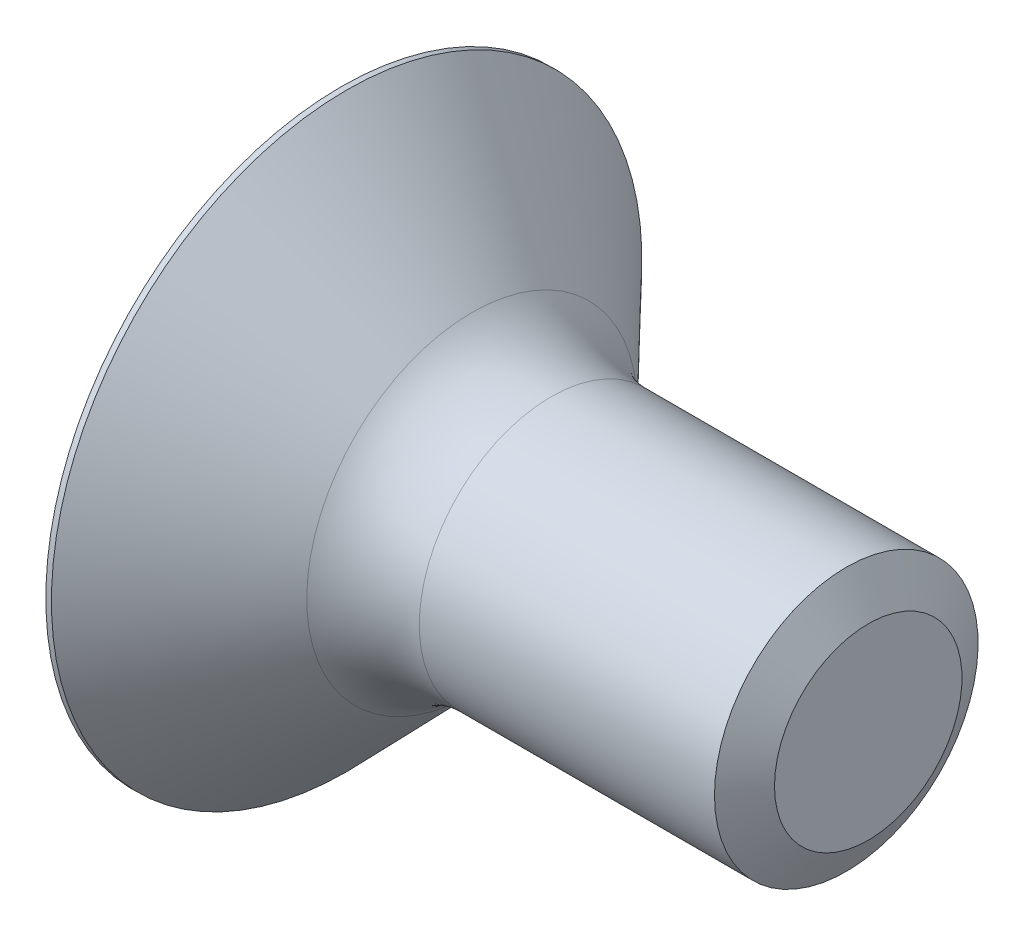
from build123d import *

# Parameters (mm, degrees)
CUT_EXTRUDE1_DEPTH = 3.82


with BuildPart() as part:
    # Sketch1 → Revolve1 (revolve)
    with BuildSketch(Plane.XY):
        with BuildLine():
            Line((0, 3), (-7.218812959, 3))
            ThreePointArc((-7.218812959, 3), (-8.195640781, 3.198737866), (-9.01716246, 3.763354074))
            Line((-9.01716246, 3.763354074), (-11.872362242, 6.72))
            Line((-11.872362242, 6.72), (-12, 6.72))
            Line((-12, 6.72), (-12, 0))
            Line((-12, 0), (0, 0))
            Line((0, 0), (0, 3))
        make_face()
    revolve(axis=Axis((0, 0, 0), (-1, 0, 0)))

    # Sketch2 → Cut-Extrude1 (cut)
    with BuildSketch(Plane.ZY.offset(12)):
        Polygon((0, 2.309401077), (-2, 1.154700538), (-2, -1.154700538), (0, -2.309401077), (2, -1.154700538), (2, 1.154700538), align=None)
    extrude(amount=-CUT_EXTRUDE1_DEPTH, mode=Mode.SUBTRACT)

    # Sketch6 → Revolve2 (revolve)
    with BuildSketch(Plane.XY, mode=Mode.PRIVATE) as revolve2_sk:
        Polygon((-9.8, 2.309401077), (-8.466666667, 0), (-7.6, 0), (-7.6, 2.309401077), align=None)
    revolve(revolve2_sk.sketch.rotate(Axis((-12, 0, 0), (1, 0, 0)), 90), axis=Axis((-12, 0, 0), (1, 0, 0)))

    # Sketch7 → Cut-Revolve2 (revolve, cut)
    with BuildSketch(Plane.XY, mode=Mode.PRIVATE) as cut_revolve2_sk:
        Polygon((-12, 2.309401077), (-12, 0), (-11.362, 0), align=None)
    revolve(cut_revolve2_sk.sketch.rotate(Axis((-12, 0, 0), (1, 0, 0)), 90), axis=Axis((-12, 0, 0), (1, 0, 0)), mode=Mode.SUBTRACT)

    # Sketch4 → Cut-Revolve1 (revolve, cut)
    with BuildSketch(Plane.XY, mode=Mode.PRIVATE) as cut_revolve1_sk:
        Polygon((-0.5, 3), (0, 2.133974596), (0.5, 3), align=None)
    revolve(cut_revolve1_sk.sketch.rotate(Axis((-0.5, 0, 0), (1, 0, 0)), 90), axis=Axis((-0.5, 0, 0), (1, 0, 0)), mode=Mode.SUBTRACT)


solid = part.part
